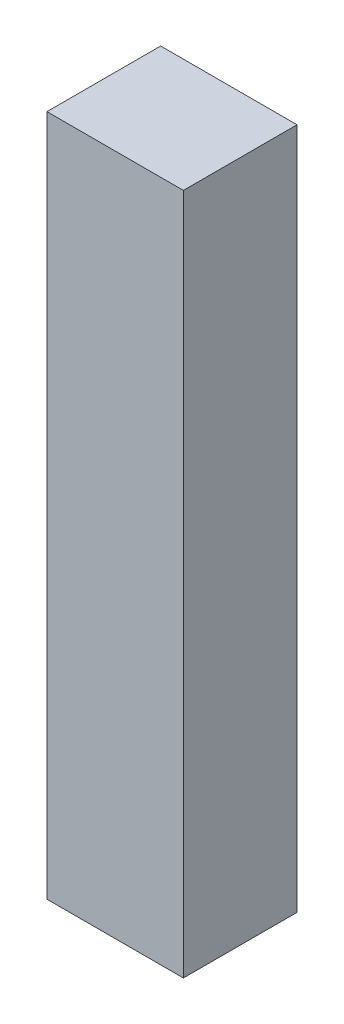
SolidWorks part; units mm, degrees
ref_plane "Front Plane" through (0, 0, 0) normal (0, 0, 1) x (1, 0, 0)
ref_plane "Top Plane" through (0, 0, 0) normal (0, 1, 0) x (1, 0, 0)
ref_plane "Right Plane" through (0, 0, 0) normal (1, 0, 0) x (0, 0, -1)
sketch "Sketch1" plane through (0, 0, 0) normal (0, 0, 1) x (1, 0, 0)
  line L1 (-43.6655, 38.7692) -> (-31.6655, 38.7692)
  line L2 (-43.6655, 38.7692) -> (-43.6655, -21.2308)
  line L3 (-43.6655, -21.2308) -> (-31.6655, -21.2308)
  line L4 (-31.6655, 38.7692) -> (-31.6655, -21.2308)
  dimension "D1" = 12
  dimension "D2" = 60
extrude "Boss-Extrude1" add sketch "Sketch1" along normal blind 10
